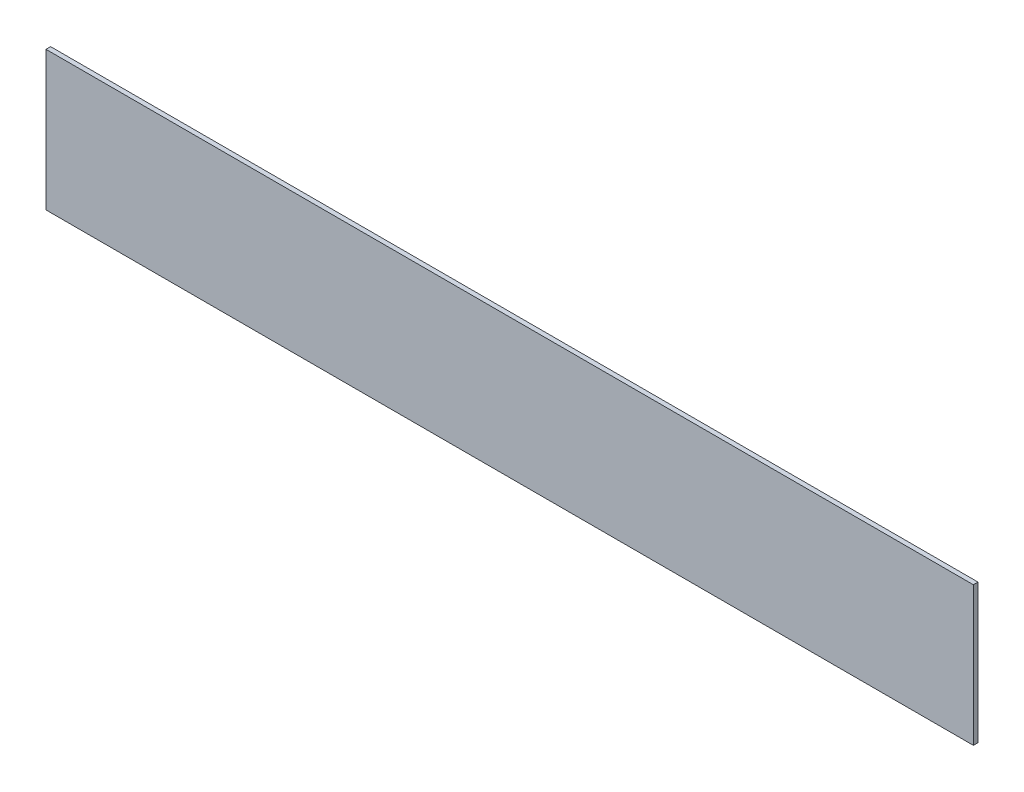
from build123d import *

# Parameters (mm, degrees)
SKETCH1_W           = 2000
SKETCH1_H           = 300
BOSS_EXTRUDE1_DEPTH = 10


with BuildPart() as part:
    # Sketch1 → Boss-Extrude1 (new body)
    with BuildSketch(Plane.XY):
        Rectangle(SKETCH1_W, SKETCH1_H)
    extrude(amount=BOSS_EXTRUDE1_DEPTH)


solid = part.part
